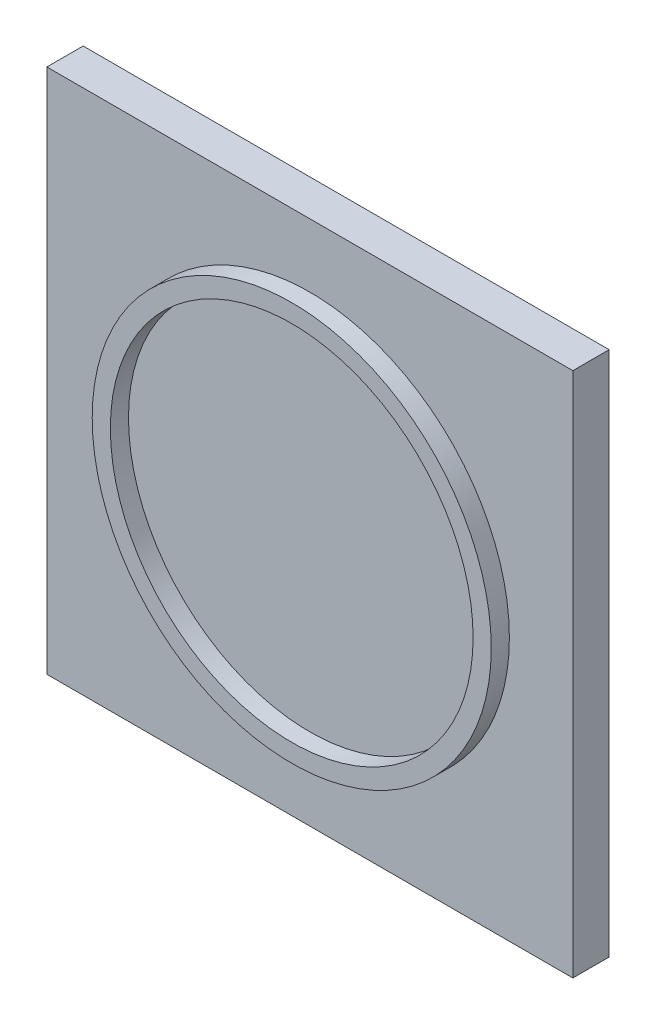
SolidWorks part; units mm, degrees
material "普通碳钢"
ref_plane "Front Plane" through (0, 0, 0) normal (0, 0, 1) x (1, 0, 0)
ref_plane "Top Plane" through (0, 0, 0) normal (0, 1, 0) x (1, 0, 0)
ref_plane "Right Plane" through (0, 0, 0) normal (1, 0, 0) x (0, 0, -1)
sketch "Sketch1" plane through (0, 0, 0) normal (0, 0, 1) x (1, 0, 0)
  line L0 (0, 0) -> (145, 0)
  line L1 (0, 0) -> (0, 145)
  line L2 (0, 145) -> (145, 145)
  line L3 (145, 145) -> (145, 0)
  dimension "D1" = 145
  dimension "D2" = 145
extrude "Boss-Extrude1" add sketch "Sketch1" along normal blind 10
sketch "Sketch2" plane through (0, 0, 10) normal (0, 0, 1) x (1, 0, 0)
  line L0 (0, 72.5) -> (145, 72.5) construction
  line L1 (0, 145) -> (0, 0) construction
  line L2 (145, 0) -> (145, 145) construction
  circle A0 centre (72.5, 72.5) radius 55
  circle A1 centre (72.5, 72.5) radius 50
  dimension "D1" = 110
  dimension "D2" = 100
extrude "Boss-Extrude2" add sketch "Sketch2" along normal blind 5
